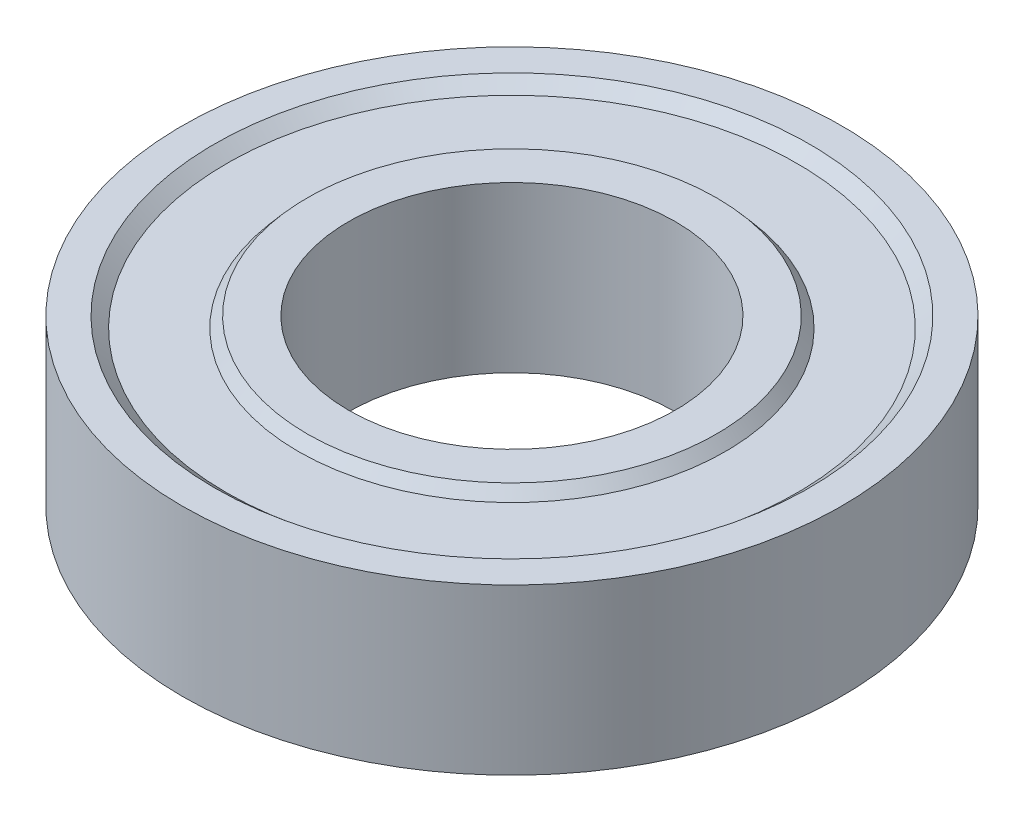
from build123d import *


with BuildPart() as part:
    # 草图1 → 旋转1 (revolve)
    with BuildSketch(Plane.XY, mode=Mode.PRIVATE) as revolve_1_sk:
        Polygon((5.95, 3), (5.95, -3), (7.45, -3), (7.779393861, -2.61408735), (10.385769976, -2.61408735), (10.837899147, -3), (12, -3), (12, 3), (10.837899147, 3), (10.385769976, 2.61408735), (7.779393861, 2.61408735), (7.45, 3), align=None)
    revolve(revolve_1_sk.sketch.rotate(Axis((0, 19.601235698, 0), (0, -1, 0)), 90), axis=Axis((0, 19.601235698, 0), (0, -1, 0)))


solid = part.part
